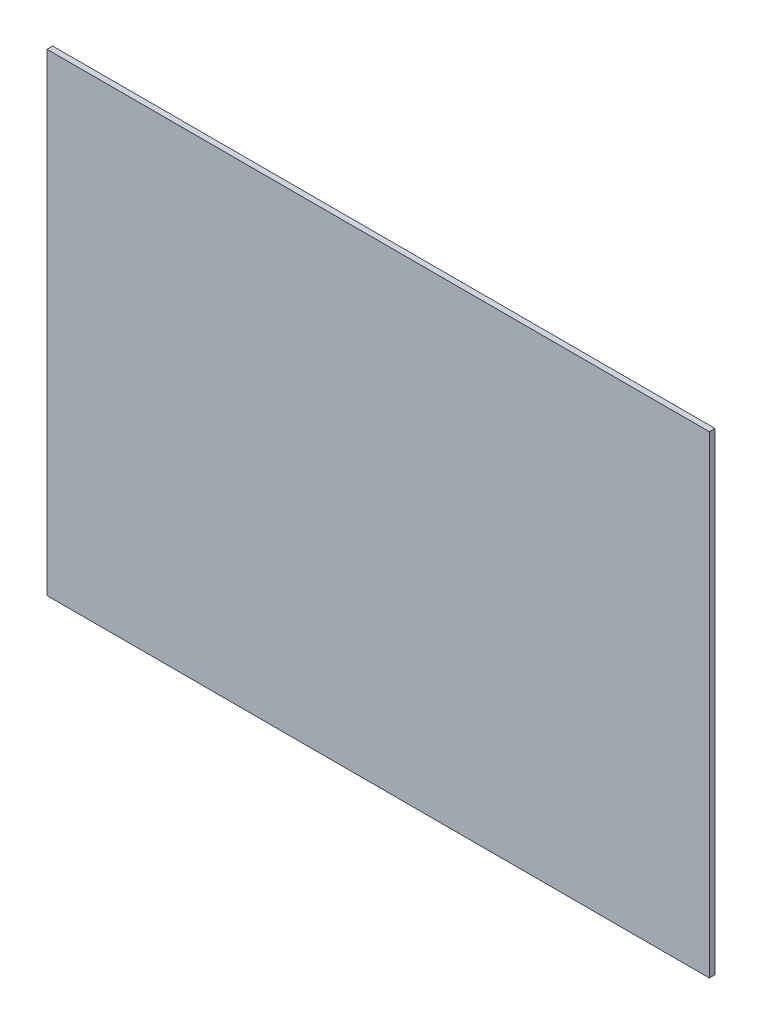
SolidWorks part; units mm, degrees
ref_plane "Front Plane" through (0, 0, 0) normal (0, 0, 1) x (1, 0, 0)
ref_plane "Top Plane" through (0, 0, 0) normal (0, 1, 0) x (1, 0, 0)
ref_plane "Right Plane" through (0, 0, 0) normal (1, 0, 0) x (0, 0, -1)
sketch "Sketch1" plane through (0, 0, 0) normal (0, 0, 1) x (1, 0, 0)
  line L1 (-350, -250) -> (350, -250)
  line L2 (-350, -250) -> (-350, 250)
  line L3 (-350, 250) -> (350, 250)
  line L4 (350, -250) -> (350, 250)
  line L5 (-350, -250) -> (350, 250) construction
  line L6 (-350, 250) -> (350, -250) construction
  point P0 (0, 0)
  dimension "D1" = 700
  dimension "D2" = 500
extrude "Boss-Extrude1" add sketch "Sketch1" along normal mid plane 6
